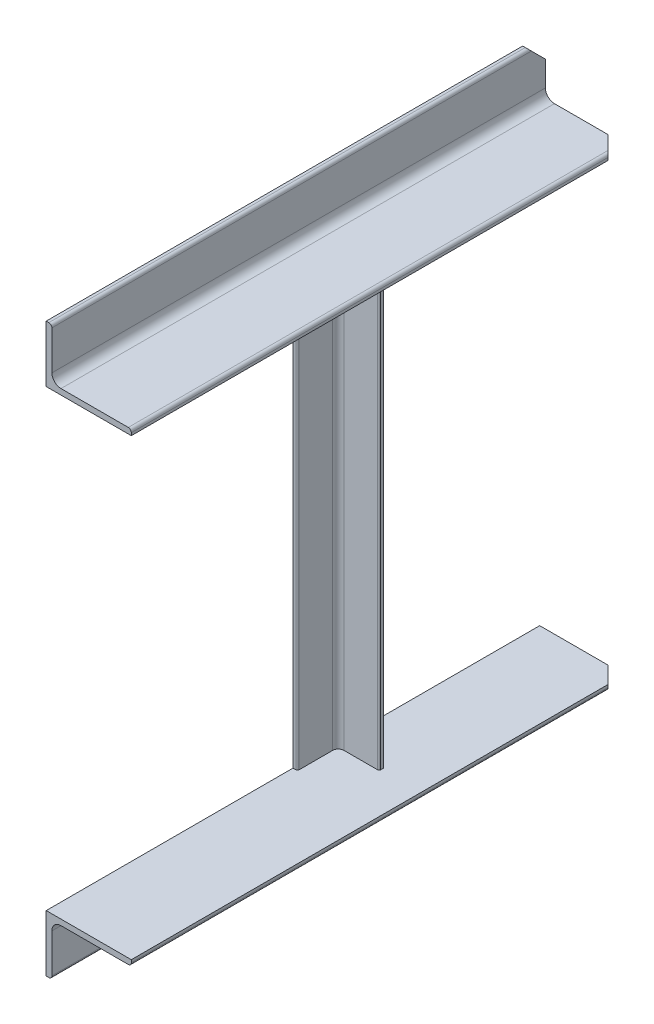
from build123d import *

# Parameters (mm, degrees)
GBT706_2008_075_50_5_1_DEPTH = 435
CUT_EXTRUDE_1_DEPTH          = 236.438420824
CUT_EXTRUDE_1_DEPTH_BACK     = 10
CUT_EXTRUDE_2_DEPTH          = 236.438420824
CUT_EXTRUDE_2_DEPTH_BACK     = 10
GBT706_2008_040_4_1_DEPTH    = 400


with BuildPart() as part:
    # Sketch12 → Gbt706-2008 热轧不等边角钢 075×50×5(1) (new body)
    with BuildSketch(Plane.YX.offset(-217.5)):
        with BuildLine():
            Line((0, 0), (0, 75))
            Line((0, 75), (2.333333333, 75))
            ThreePointArc((2.333333333, 75), (4.218951416, 74.218951416), (5, 72.333333333))
            Line((5, 72.333333333), (5, 13))
            ThreePointArc((5, 13), (7.343145751, 7.343145751), (13, 5))
            Line((13, 5), (47.333333333, 5))
            ThreePointArc((47.333333333, 5), (49.218951416, 4.218951416), (50, 2.333333333))
            Line((50, 2.333333333), (50, 0))
            Line((50, 0), (0, 0))
        make_face()
    extrude(amount=GBT706_2008_075_50_5_1_DEPTH)

    # 草图2 → 切除-拉伸1 (cut, two sides: drawn at the far end of the back side and taken through both)
    with BuildSketch(Plane.ZY.offset(-CUT_EXTRUDE_1_DEPTH_BACK)):
        Polygon((-841.74203278, -589.24203278), (-217.5, 35), (-202.5, 50), (421.74203278, 674.24203278), (-826.74203278, 1922.726098341), (-2090.226098341, 659.24203278), align=None)
    extrude(amount=CUT_EXTRUDE_1_DEPTH + CUT_EXTRUDE_1_DEPTH_BACK, mode=Mode.SUBTRACT)

    # 草图3 → 切除-拉伸2 (cut, two sides: drawn at the far end of the back side and taken through both)
    with BuildSketch(Plane.XZ.offset(-CUT_EXTRUDE_2_DEPTH_BACK)):
        Polygon((-568.078314146, -845.578314146), (60, -217.5), (75, -202.5), (703.078314146, 425.578314146), (1959.234942439, -830.578314146), (688.078314146, -2101.734942439), align=None)
    extrude(amount=CUT_EXTRUDE_2_DEPTH + CUT_EXTRUDE_2_DEPTH_BACK, mode=Mode.SUBTRACT)


with BuildPart() as body_2:
    # 镜向2: mirrored copy
    add(part.part.mirror(Plane(origin=(0, -200, 0), x_dir=(0, 0, 1), z_dir=(0, -1, 0))))


with BuildPart() as body_3:
    # Sketch15 → Gbt706-2008 热轧等边角钢 040×4(1) (new body)
    with BuildSketch(Plane(origin=(0, 0, -40), x_dir=(0, 0, 1), z_dir=(0, 1, 0))):
        with BuildLine():
            Line((0, 0), (0, 40))
            Line((0, 40), (2.666666667, 40))
            ThreePointArc((2.666666667, 40), (3.609475708, 39.609475708), (4, 38.666666667))
            Line((4, 38.666666667), (4, 9))
            ThreePointArc((4, 9), (5.464466094, 5.464466094), (9, 4))
            Line((9, 4), (38.666666667, 4))
            ThreePointArc((38.666666667, 4), (39.609475708, 3.609475708), (40, 2.666666667))
            Line((40, 2.666666667), (40, 0))
            Line((40, 0), (0, 0))
        make_face()
    extrude(amount=-GBT706_2008_040_4_1_DEPTH)


solid = Compound([part.part, body_2.part, body_3.part])
